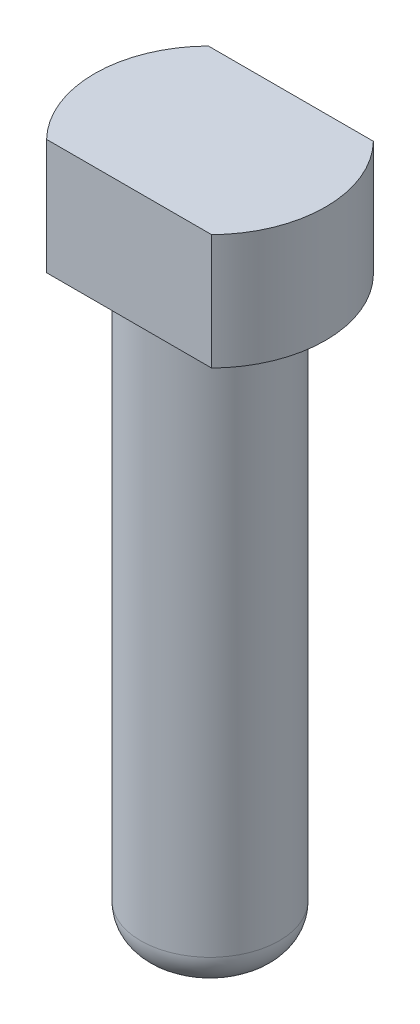
SolidWorks part; units mm, degrees
material "6061"
ref_plane "前视基准面" through (0, 0, 0) normal (0, 0, 1) x (1, 0, 0)
ref_plane "上视基准面" through (0, 0, 0) normal (0, 1, 0) x (1, 0, 0)
ref_plane "右视基准面" through (0, 0, 0) normal (1, 0, 0) x (0, 0, -1)
sketch "草图1" plane through (0, 0, 0) normal (0, 1, 0) x (1, 0, 0)
  circle A0 centre (0, 0) radius 10
  dimension "D1" = 20
extrude "凸台-拉伸1" add sketch "草图1" along normal mid plane 60
sketch "草图2" plane through (0, -30, 0) normal (0, -1, 0) x (1, 0, 0)
  circle A0 centre (0, 0) radius 6
  circle A1 centre (0, 0) radius 10
  circle A2 centre (0, 0) radius 10 construction
  dimension "D1" = 12
extrude "切除-拉伸1" cut sketch "草图2" against normal blind 50
fillet "圆角1" radius 3 1 edges at (0, -30, -6)
sketch "草图3" plane through (0, 30, 0) normal (0, 1, 0) x (1, 0, 0)
  line L0 (-12.1489, 0) -> (13.2483, 0) construction
  line L1 (-7.1414, 7) -> (7.1414, 7)
  line L3 (-7.1414, -7) -> (7.1414, -7)
  circle A0 centre (0, 0) radius 10 construction
  arc A1 (-7.1414, -7) -> (7.1414, -7) centre (0, 0) ccw
  arc A2 (7.1414, 7) -> (-7.1414, 7) centre (0, 0) ccw
  point P0 (0, 0)
  dimension "D1" = 14
extrude "切除-拉伸3" cut sketch "草图3" against normal blind 10
